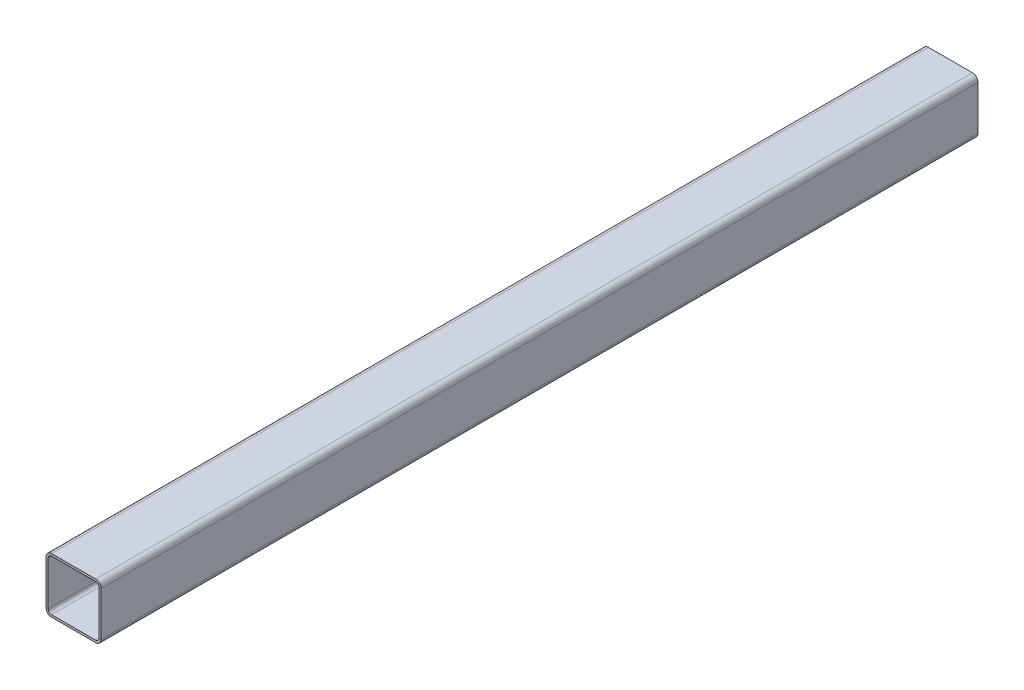
SolidWorks part; units mm, degrees
ref_plane "Front Plane" through (0, 0, 0) normal (0, 0, 1) x (1, 0, 0)
ref_plane "Top Plane" through (0, 0, 0) normal (0, 1, 0) x (1, 0, 0)
ref_plane "Right Plane" through (0, 0, 0) normal (1, 0, 0) x (0, 0, -1)
other "Configuration Table"
sketch "Sketch1" plane through (0, 0, 0) normal (0, 0, 1) x (1, 0, 0)
  line L0 (-92, 80) -> (-92, -80)
  line L1 (-80, 100) -> (80, 100)
  line L2 (-100, 80) -> (-100, -80)
  line L3 (-80, -100) -> (80, -100)
  line L4 (100, 80) -> (100, -80)
  line L5 (-100, 100) -> (100, -100) construction
  line L6 (-100, -100) -> (100, 100) construction
  line L7 (-80, -92) -> (80, -92)
  line L8 (92, 80) -> (92, -80)
  line L9 (-80, 92) -> (80, 92)
  arc A0 (-100, -80) -> (-80, -100) centre (-80, -80) ccw
  arc A1 (80, -100) -> (100, -80) centre (80, -80) ccw
  arc A2 (80, 100) -> (100, 80) centre (80, 80) cw
  arc A3 (-80, 100) -> (-100, 80) centre (-80, 80) ccw
  arc A4 (-92, -80) -> (-80, -92) centre (-80, -80) ccw
  arc A5 (80, -92) -> (92, -80) centre (80, -80) ccw
  arc A6 (80, 92) -> (92, 80) centre (80, 80) cw
  arc A7 (-80, 92) -> (-92, 80) centre (-80, 80) ccw
  point P0 (0, 0)
  dimension "D3" = 20
  dimension "D1" = 200
  dimension "D2" = 200
  dimension "D4" = 8
extrude "Boss-Extrude1" add sketch "Sketch1" along normal blind 3180
